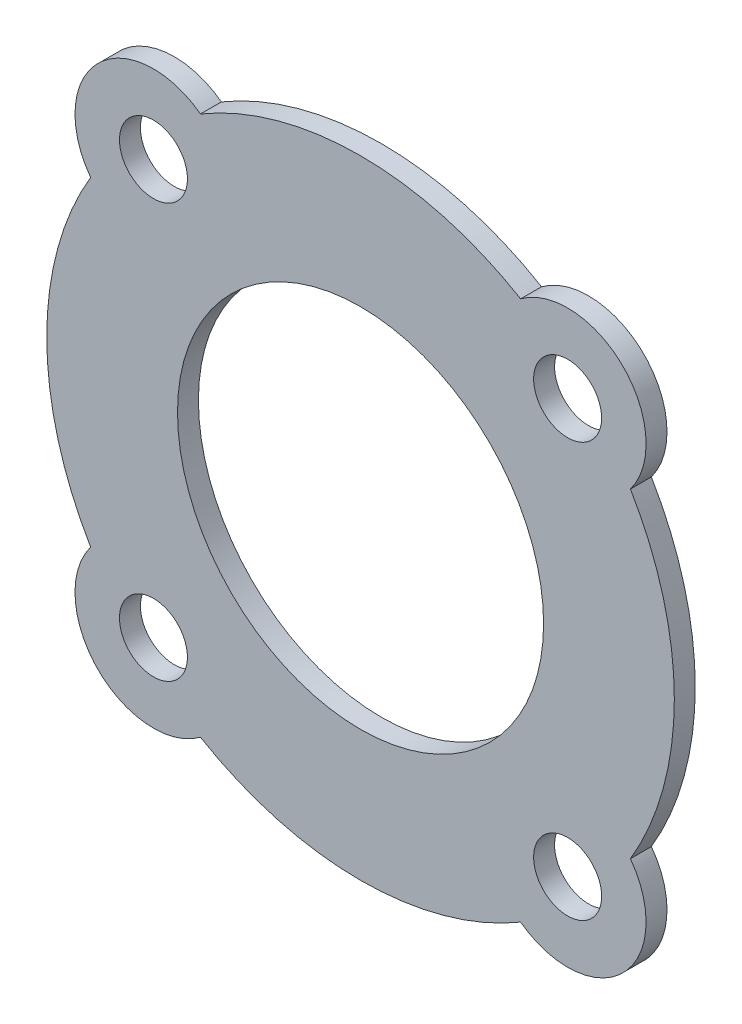
from build123d import *

# Parameters (mm, degrees)
SKETCH1_R           = 35
SKETCH1_R_2         = 6.5
BOSS_EXTRUDE1_DEPTH = 2


with BuildPart() as part:
    # Sketch1 → Boss-Extrude1 (new, symmetric)
    with BuildSketch(Plane.XY):
        with BuildLine():
            ThreePointArc((30.608172596, 51.605617624), (0, 60), (-30.608172596, 51.605617624))
            ThreePointArc((-30.608172596, 51.605617624), (-50.204581464, 50.204581464), (-51.605617624, 30.608172596))
            ThreePointArc((-51.605617624, 30.608172596), (-60, 0), (-51.605617624, -30.608172596))
            ThreePointArc((-51.605617624, -30.608172596), (-50.204581464, -50.204581464), (-30.608172596, -51.605617624))
            ThreePointArc((-30.608172596, -51.605617624), (0, -60), (30.608172596, -51.605617624))
            ThreePointArc((30.608172596, -51.605617624), (50.204581464, -50.204581464), (51.605617624, -30.608172596))
            ThreePointArc((51.605617624, -30.608172596), (60, 0), (51.605617624, 30.608172596))
            ThreePointArc((51.605617624, 30.608172596), (50.204581464, 50.204581464), (30.608172596, 51.605617624))
        make_face()
        Circle(SKETCH1_R, mode=Mode.SUBTRACT)
        with Locations((39.597979746, 39.597979746)):
            Circle(SKETCH1_R_2, mode=Mode.SUBTRACT)
        with Locations((39.597979746, -39.597979746)):
            Circle(SKETCH1_R_2, mode=Mode.SUBTRACT)
        with Locations((-39.597979746, -39.597979746)):
            Circle(SKETCH1_R_2, mode=Mode.SUBTRACT)
        with Locations((-39.597979746, 39.597979746)):
            Circle(SKETCH1_R_2, mode=Mode.SUBTRACT)
    extrude(amount=BOSS_EXTRUDE1_DEPTH, both=True)


solid = part.part
